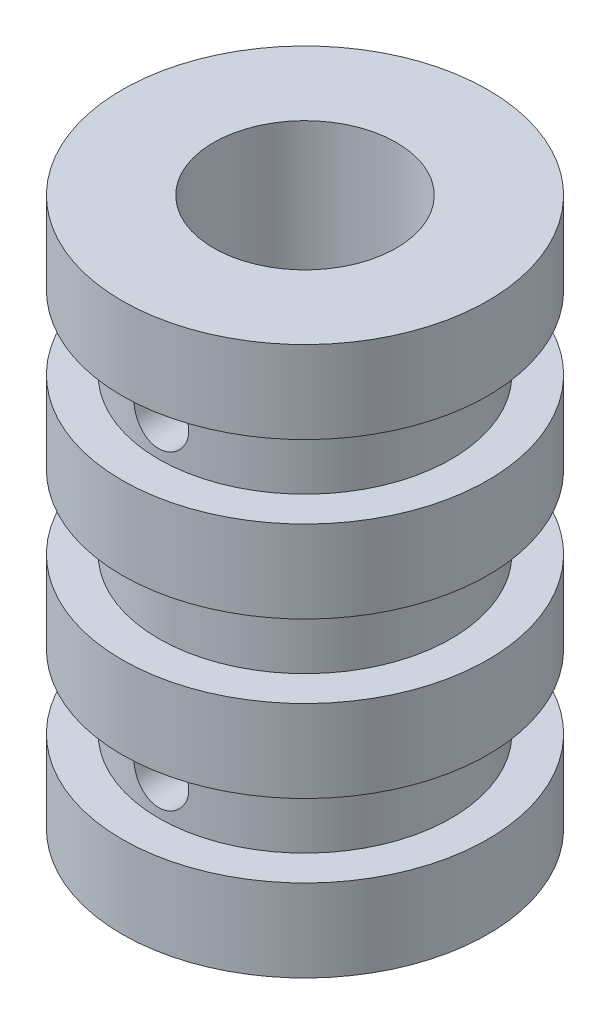
from build123d import *

# Parameters (mm, degrees)
CUT_EXTRUDE1_REACH      = 35.166
CUT_EXTRUDE1_END_RADIUS = 8
SKETCH2_R               = 1.5


with BuildPart() as part:
    # Sketch1 → Revolve1 (revolve)
    with BuildSketch(Plane.XY, mode=Mode.PRIVATE) as revolve1_sk:
        Polygon((2.5, 15), (2.5, 0), (10, 0), (10, 4.5), (8, 4.5), (8, 8.5), (10, 8.5), (10, 13), (8, 13), (8, 17), (10, 17), (10, 21.5), (8, 21.5), (8, 25.5), (10, 25.5), (10, 30), (5, 30), (5, 15), align=None)
    revolve(revolve1_sk.sketch.rotate(Axis((0, 0, 0), (0, 1, 0)), 90), axis=Axis((0, 0, 0), (0, 1, 0)))

    # Cut-Extrude1: up to this cylinder (the profile starts inside it)
    cut_extrude1_end = Plane(origin=(0, 15, 0), z_dir=(0, -1, 0)) * Cylinder(CUT_EXTRUDE1_END_RADIUS, 104.332, mode=Mode.PRIVATE)
    # Sketch2 → Cut-Extrude1 (cut, up to the surface)
    with BuildSketch(Plane.XY, mode=Mode.PRIVATE) as cut_extrude1_sk1:
        with Locations(Location((0, 23.5, 0), (0, 0, 180))):
            Circle(SKETCH2_R)
    cut_extrude1_tool1 = extrude(cut_extrude1_sk1.sketch, amount=CUT_EXTRUDE1_REACH, mode=Mode.PRIVATE) & cut_extrude1_end
    add(cut_extrude1_tool1.solids().sort_by_distance((0, 23.5, 0))[0], mode=Mode.SUBTRACT)
    # Sketch2 → Cut-Extrude1 (cut, up to the surface)
    with BuildSketch(Plane.XY, mode=Mode.PRIVATE) as cut_extrude1_sk2:
        with Locations(Location((0, 6.5, 0), (0, 0, 180))):
            Circle(SKETCH2_R)
    cut_extrude1_tool2 = extrude(cut_extrude1_sk2.sketch, amount=CUT_EXTRUDE1_REACH, mode=Mode.PRIVATE) & cut_extrude1_end
    add(cut_extrude1_tool2.solids().sort_by_distance((0, 6.5, 0))[0], mode=Mode.SUBTRACT)


solid = part.part
